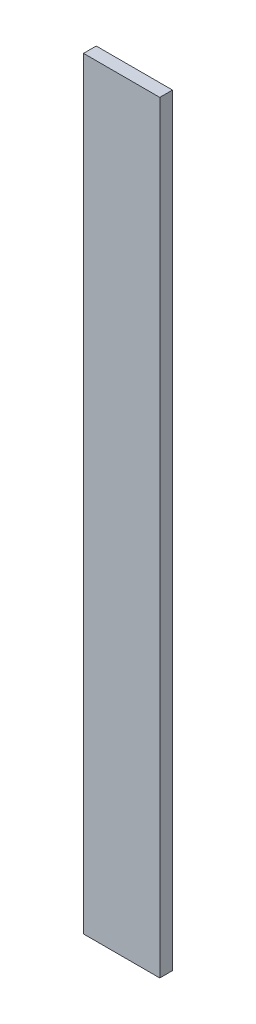
SolidWorks part; units mm, degrees
material "Q235"
ref_plane "Front Plane" through (0, 0, 0) normal (0, 0, 1) x (1, 0, 0)
ref_plane "Top Plane" through (0, 0, 0) normal (0, 1, 0) x (1, 0, 0)
ref_plane "Right Plane" through (0, 0, 0) normal (1, 0, 0) x (0, 0, -1)
sketch "Sketch1" plane through (0, 0, 0) normal (0, 0, 1) x (1, 0, 0)
  line L1 (0, 0) -> (60, 0)
  line L2 (0, 0) -> (0, 600)
  line L3 (0, 600) -> (60, 600)
  line L4 (60, 0) -> (60, 600)
  dimension "D1" = 60
  dimension "D2" = 600
extrude "Boss-Extrude1" add sketch "Sketch1" along normal blind 10
